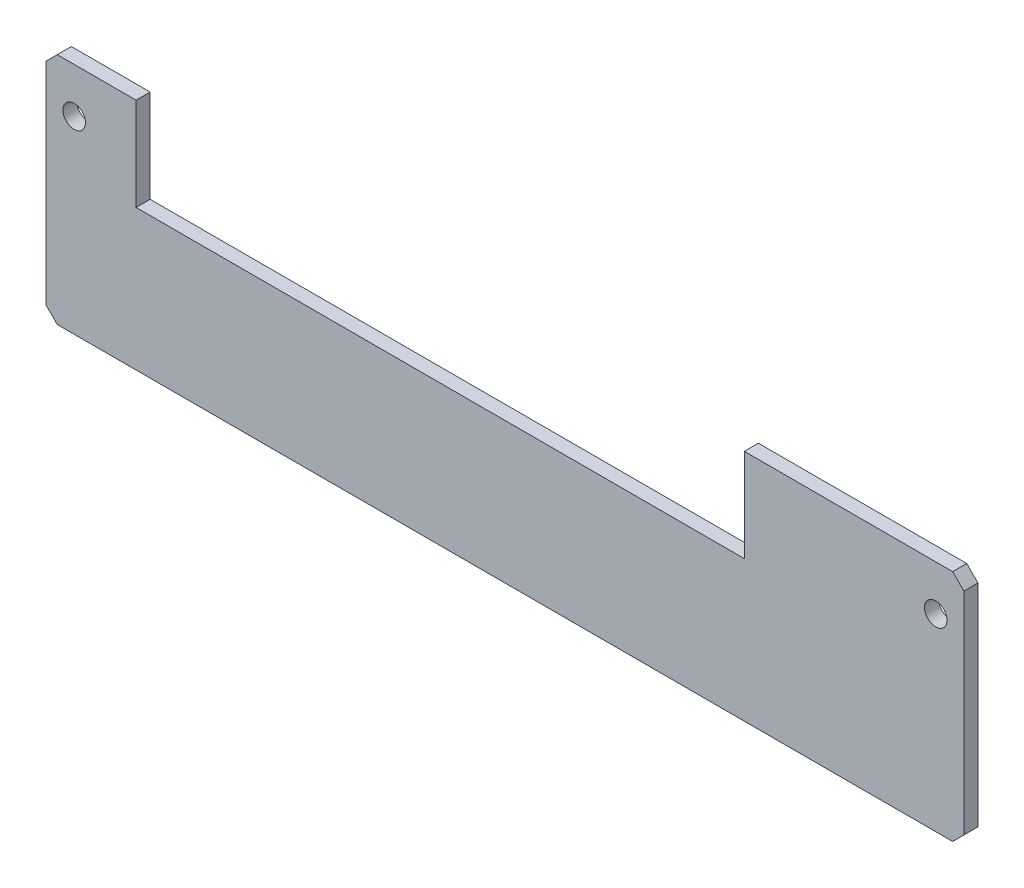
SolidWorks part; units mm, degrees
ref_plane "Front Plane" through (0, 0, 0) normal (0, 0, 1) x (1, 0, 0)
ref_plane "Top Plane" through (0, 0, 0) normal (0, 1, 0) x (1, 0, 0)
ref_plane "Right Plane" through (0, 0, 0) normal (1, 0, 0) x (0, 0, -1)
sketch "Sketch1" plane through (0, 0, 0) normal (0, 0, 1) x (1, 0, 0)
  line L1 (815, 207.5) -> (-815, 207.5)
  line L2 (815, 207.5) -> (815, -207.5)
  line L3 (815, -207.5) -> (-815, -207.5)
  line L4 (-815, 207.5) -> (-815, -207.5)
  line L5 (815, 207.5) -> (-815, -207.5) construction
  line L6 (815, -207.5) -> (-815, 207.5) construction
  point P0 (0, 0)
  dimension "D1" = 1630
  dimension "D2" = 415
extrude "Boss-Extrude1" add sketch "Sketch1" along normal blind 25
chamfer "Chamfer1" distance 20 angle 45 4 edges at (-815, -207.5, 12.5) (815, -207.5, 12.5) (815, 207.5, 12.5) (-815, 207.5, 12.5)
sketch "Sketch2" plane through (0, 0, 25) normal (0, 0, 1) x (1, 0, 0)
  line L5 (-815, 187.5) -> (-815, -187.5) construction
  line L6 (795, 207.5) -> (-795, 207.5) construction
  line L7 (815, -187.5) -> (815, 187.5) construction
  line L8 (-655, 42.5) -> (425, 42.5)
  line L9 (-655, 42.5) -> (-655, 242.5)
  line L10 (-655, 242.5) -> (425, 242.5)
  line L11 (425, 42.5) -> (425, 242.5)
  circle A0 centre (-765, 127.5) radius 20
  circle A1 centre (765, 127.5) radius 20
  dimension "D8" = 40
  dimension "D4" = 50
  dimension "D5" = 80
  dimension "D6" = 50
  dimension "D7" = 80
extrude "Cut-Extrude1" cut sketch "Sketch2" against normal through all both and the other way through all
